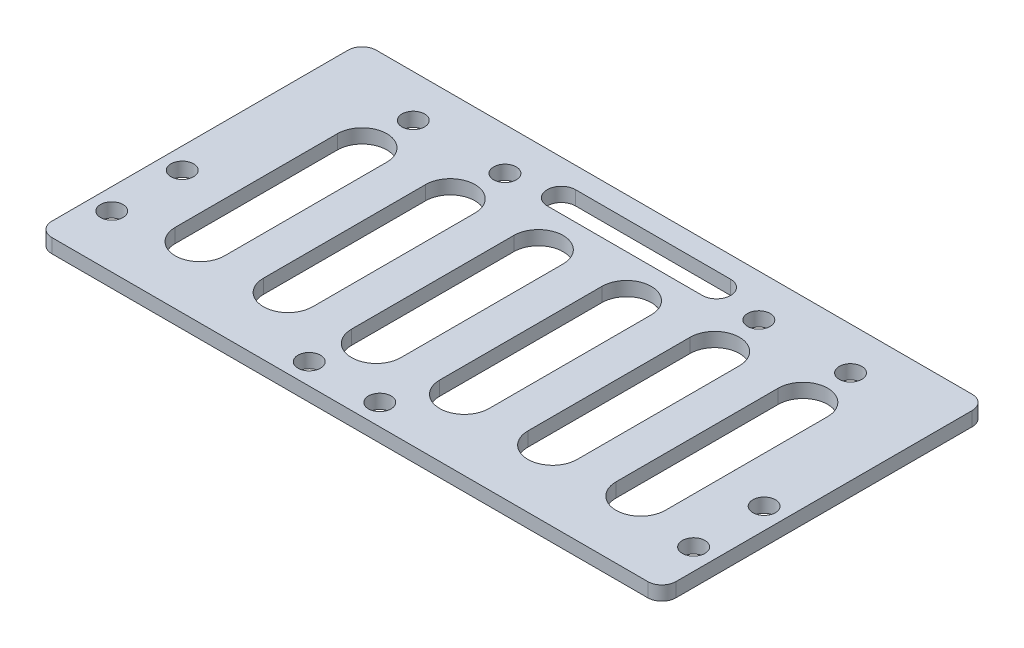
from build123d import *

# Parameters (mm, degrees)
SKETCH1_W           = 88.5
SKETCH1_H           = 46
SKETCH1_R           = 1.6
BOSS_EXTRUDE1_DEPTH = 2
CUT_EXTRUDE1_DEPTH  = 50.910544978
FILLET1_R           = 2


with BuildPart() as part:
    # Sketch1 → Boss-Extrude1 (new body)
    with BuildSketch(Plane(origin=(0, 0, 0), x_dir=(1, 0, 0), z_dir=(0, 1, 0))):
        Rectangle(SKETCH1_W, SKETCH1_H)
        with Locations(Location((-41.25, -5.5, 0), (0, 0, 270))):
            Circle(SKETCH1_R, mode=Mode.SUBTRACT)
        with Locations(Location((-41.25, -15.5, 0), (0, 0, 270))):
            Circle(SKETCH1_R, mode=Mode.SUBTRACT)
        with Locations(Location((41.25, -15.5, 0), (0, 0, 90))):
            Circle(SKETCH1_R, mode=Mode.SUBTRACT)
        with Locations(Location((41.25, -5.5, 0), (0, 0, 90))):
            Circle(SKETCH1_R, mode=Mode.SUBTRACT)
        with Locations(Location((-8.75, -20, 0), (0, 0, 270))):
            Circle(SKETCH1_R, mode=Mode.SUBTRACT)
        with Locations(Location((1.25, -20, 0), (0, 0, 270))):
            Circle(SKETCH1_R, mode=Mode.SUBTRACT)
        with Locations(Location((-31, 17, 0), (0, 0, 270))):
            Circle(SKETCH1_R, mode=Mode.SUBTRACT)
        with Locations(Location((-18, 17, 0), (0, 0, 270))):
            Circle(SKETCH1_R, mode=Mode.SUBTRACT)
        with Locations(Location((18, 17, 0), (0, 0, 270))):
            Circle(SKETCH1_R, mode=Mode.SUBTRACT)
        with Locations(Location((31, 17, 0), (0, 0, 270))):
            Circle(SKETCH1_R, mode=Mode.SUBTRACT)
    extrude(amount=BOSS_EXTRUDE1_DEPTH)

    # Sketch2 → Cut-Extrude1 (cut, through all)
    with BuildSketch(Plane(origin=(0, 2, 0), x_dir=(1, 0, 0), z_dir=(0, 1, 0))):
        with BuildLine():
            Line((-27.75, 10), (-27.75, -13))
            ThreePointArc((-27.75, -13), (-31.25, -16.5), (-34.75, -13))
            Line((-34.75, -13), (-34.75, 10))
            ThreePointArc((-34.75, 10), (-31.25, 13.5), (-27.75, 10))
        make_face()
        with BuildLine():
            Line((-15.25, 10), (-15.25, -13))
            ThreePointArc((-15.25, -13), (-18.75, -16.5), (-22.25, -13))
            Line((-22.25, -13), (-22.25, 10))
            ThreePointArc((-22.25, 10), (-18.75, 13.5), (-15.25, 10))
        make_face()
        with BuildLine():
            Line((-2.75, 10), (-2.75, -13))
            ThreePointArc((-2.75, -13), (-6.25, -16.5), (-9.75, -13))
            Line((-9.75, -13), (-9.75, 10))
            ThreePointArc((-9.75, 10), (-6.25, 13.5), (-2.75, 10))
        make_face()
        with BuildLine():
            Line((9.75, 10), (9.75, -13))
            ThreePointArc((9.75, -13), (6.25, -16.5), (2.75, -13))
            Line((2.75, -13), (2.75, 10))
            ThreePointArc((2.75, 10), (6.25, 13.5), (9.75, 10))
        make_face()
        with BuildLine():
            Line((22.25, 10), (22.25, -13))
            ThreePointArc((22.25, -13), (18.75, -16.5), (15.25, -13))
            Line((15.25, -13), (15.25, 10))
            ThreePointArc((15.25, 10), (18.75, 13.5), (22.25, 10))
        make_face()
        with BuildLine():
            Line((34.75, 10), (34.75, -13))
            ThreePointArc((34.75, -13), (31.25, -16.5), (27.75, -13))
            Line((27.75, -13), (27.75, 10))
            ThreePointArc((27.75, 10), (31.25, 13.5), (34.75, 10))
        make_face()
        with BuildLine():
            Line((-11, 20), (11, 20))
            ThreePointArc((11, 20), (13, 18), (11, 16))
            Line((11, 16), (-11, 16))
            ThreePointArc((-11, 16), (-13, 18), (-11, 20))
        make_face()
    extrude(amount=-CUT_EXTRUDE1_DEPTH, mode=Mode.SUBTRACT)

    # Fillet1
    fillet1_edges = [part.edges().sort_by_distance(p)[0] for p in [
        (44.25, 1, 23),
        (-44.25, 1, 23),
        (-44.25, 1, -23),
        (44.25, 1, -23),
    ]]
    fillet(fillet1_edges, radius=FILLET1_R)


solid = part.part
